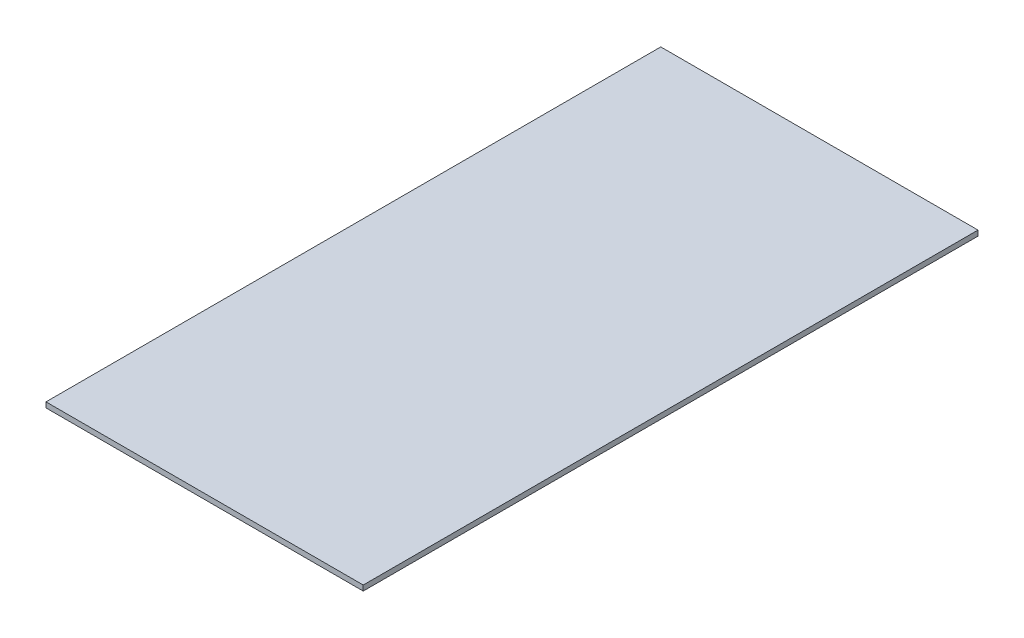
from build123d import *

# Parameters (mm, degrees)
SKETCH_1_W      = 903
SKETCH_1_H      = 1750
EXTRUDE_1_DEPTH = 15


with BuildPart() as part:
    # 草图1 → 凸台-拉伸1 (new body)
    with BuildSketch(Plane(origin=(0, 0, 0), x_dir=(1, 0, 0), z_dir=(0, 1, 0))):
        with Locations((451.5, -875)):
            Rectangle(SKETCH_1_W, SKETCH_1_H)
    extrude(amount=EXTRUDE_1_DEPTH)


solid = part.part
